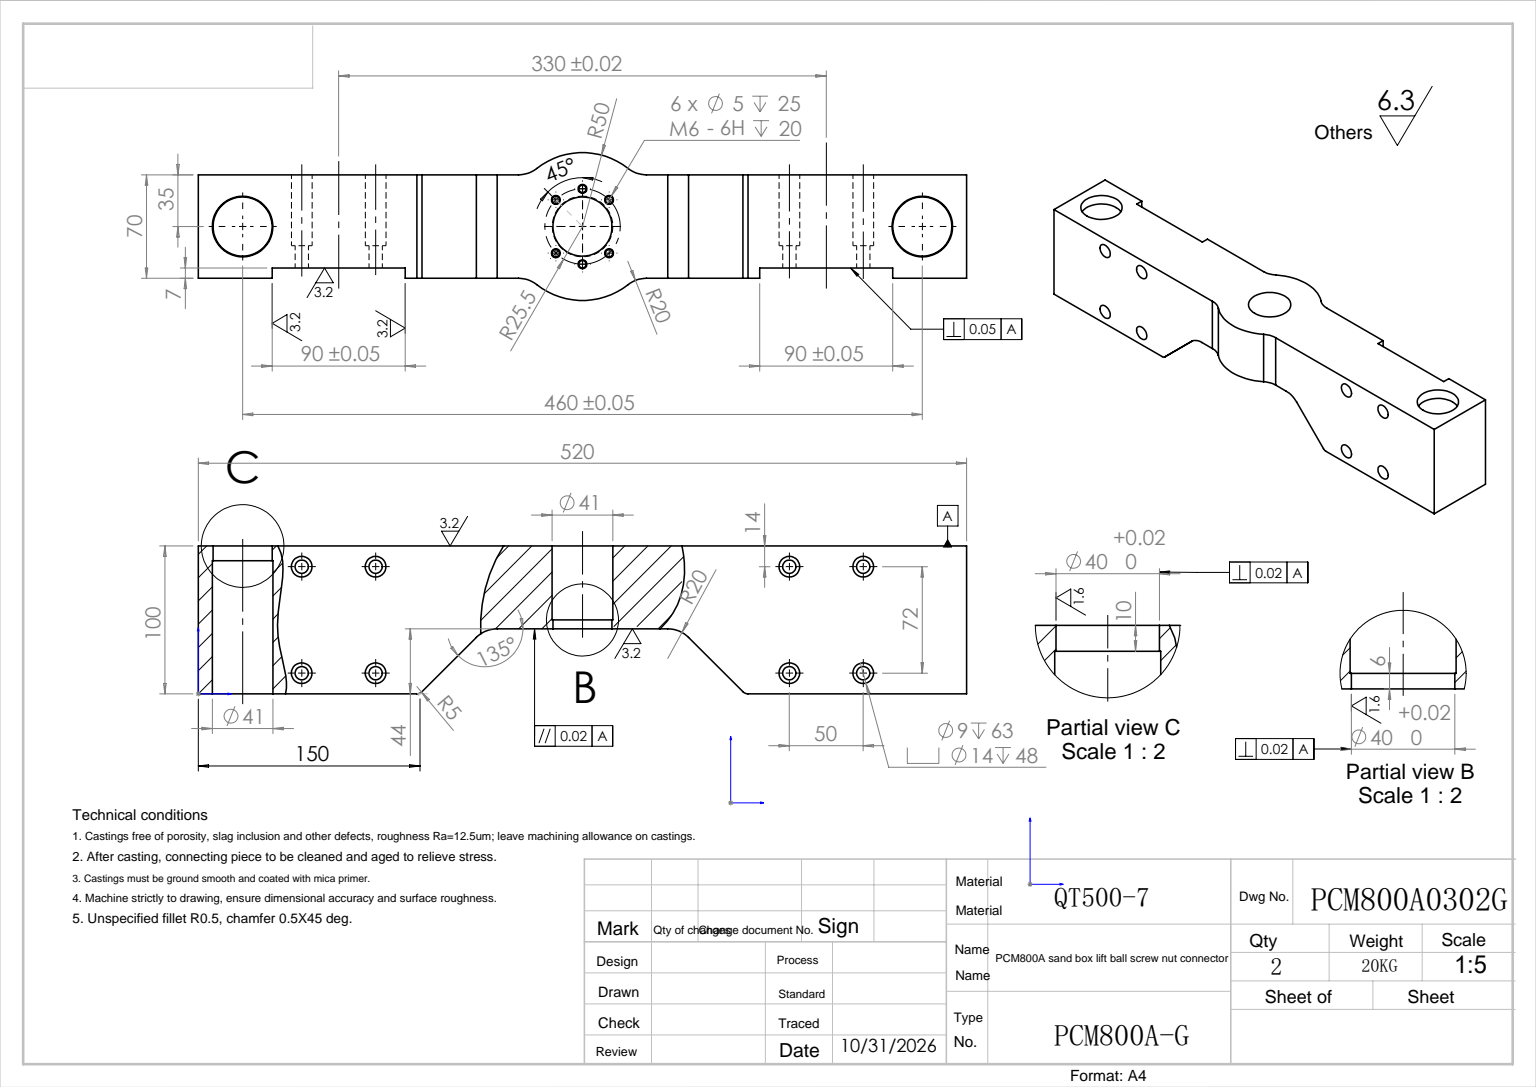
SolidWorks part; units mm, degrees
material "灰铸铁"
ref_plane "前视基准面" through (0, 0, 0) normal (0, 0, 1) x (1, 0, 0)
ref_plane "上视基准面" through (0, 0, 0) normal (0, 1, 0) x (1, 0, 0)
ref_plane "右视基准面" through (0, 0, 0) normal (1, 0, 0) x (0, 0, -1)
sketch "草图1" plane through (0, 0, 0) normal (0, 1, 0) x (1, 0, 0)
  line L0 (0, 70) -> (0, 0)
  line L1 (520, 70) -> (520, 0)
  line L5 (0, 70) -> (50, 70)
  line L6 (50, 70) -> (50, 63)
  line L7 (50, 63) -> (140, 63)
  line L8 (0, 0) -> (216.6987, 0)
  line L9 (260, 0) -> (260, 88.2574) construction
  line L10 (140, 63) -> (140, 70)
  line L11 (140, 70) -> (216.6987, 70)
  line L12 (380, 63) -> (380, 70)
  line L13 (470, 63) -> (380, 63)
  line L14 (470, 70) -> (470, 63)
  line L15 (520, 70) -> (470, 70)
  line L21 (260, 35) -> (280.0863, 35) construction
  line L22 (303.3013, 70) -> (380, 70)
  line L23 (303.3013, 0) -> (520, 0)
  arc A0 (229.0705, -4.2857) -> (290.9295, -4.2857) centre (260, 35) ccw
  arc A1 (290.9295, 74.2857) -> (229.0705, 74.2857) centre (260, 35) ccw
  arc A2 (216.6987, 70) -> (229.0705, 74.2857) centre (216.6987, 90) ccw
  arc A3 (303.3013, 70) -> (290.9295, 74.2857) centre (303.3013, 90) cw
  arc A4 (303.3013, 0) -> (290.9295, -4.2857) centre (303.3013, -20) ccw
  arc A5 (216.6987, 0) -> (229.0705, -4.2857) centre (216.6987, -20) cw
  point P15 (260, 70)
  point P34 (295.7071, 70)
  dimension "D10" = 20
  dimension "D5" = 50
  dimension "D6" = 7
  dimension "D7" = 90
  dimension "D8" = 260
  dimension "D9" = 35
extrude "拉伸1" add sketch "草图1" along normal blind 100
sketch "草图2" plane through (0, 0, 0) normal (0, 0, 1) x (1, 0, 0)
  line L0 (260, 100) -> (260, 0) construction
  line L1 (290.9295, 100) -> (229.0705, 100) construction
  line L2 (229.0705, 0) -> (290.9295, 0) construction
  line L3 (317.7158, 43.9997) -> (202.2842, 43.9997)
  line L5 (0, 0) -> (216.6987, 0) construction
  line L6 (331.8579, 38.1419) -> (370, 0)
  line L8 (188.1421, 38.1419) -> (150, 0)
  line L9 (150, 0) -> (370, 0)
  arc A0 (188.1421, 38.1419) -> (202.2842, 43.9997) centre (202.2842, 23.9997) cw
  arc A1 (331.8579, 38.1419) -> (317.7158, 43.9997) centre (317.7158, 23.9997) ccw
  point P6 (326, 43.9997)
  point P9 (194, 43.9997)
  point P13 (194, 43.9997)
  point P18 (326, 43.9997)
  point P20 (260, 43.9997)
  dimension "D3" = 56.0003
  dimension "D4" = 20
  dimension "D1" = 66
  dimension "D2" = 110
extrude "切除-拉伸1" cut sketch "草图2" against normal through all and the other way through all
sketch "草图3" plane through (0, 43.9997, 0) normal (0, -1, 0) x (1, 0, 0)
  circle A0 centre (260, -35) radius 20
extrude "切除-拉伸2" cut sketch "草图3" against normal through all
ref_plane "基准面1" through (260, 0, 0) normal (1, 0, 0) x (0, 0, -1)
sketch "草图7" plane through (0, 0, -63) normal (0, 0, -1) x (-1, 0, 0)
  line L0 (-425, 100) -> (-425, 0) construction
  line L1 (-470, 100) -> (-380, 100) construction
  line L2 (-470, 0) -> (-380, 0) construction
  line L3 (-470, 50) -> (-380, 50) construction
  line L4 (-470, 100) -> (-470, 0) construction
  line L5 (-380, 100) -> (-380, 0) construction
  line L6 (-450, 86) -> (-400, 86) construction
  line L7 (-400, 86) -> (-400, 14) construction
  line L8 (-400, 14) -> (-450, 14) construction
  line L9 (-450, 14) -> (-450, 86) construction
  circle A0 centre (-450, 86) radius 4.5
  circle A1 centre (-400, 86) radius 4.5
  circle A2 centre (-400, 14) radius 4.5
  circle A3 centre (-450, 14) radius 4.5
  dimension "D1" = 36
  dimension "D2" = 36
  dimension "D3" = 25
  dimension "D4" = 25
extrude "切除-拉伸4" cut sketch "草图7" against normal through all
sketch "草图8" plane through (0, 0, 0) normal (0, 0, 1) x (1, 0, 0)
  circle A0 centre (400, 86) radius 7
  circle A1 centre (450, 86) radius 7
  circle A2 centre (450, 14) radius 7
  circle A3 centre (400, 14) radius 7
extrude "切除-拉伸5" cut sketch "草图8" against normal blind 48
mirror "镜向2" about plane through (260, 0, 0) normal (1, 0, 0) of "切除-拉伸4", "切除-拉伸5"
sketch "草图12" plane through (0, 43.9997, 0) normal (0, -1, 0) x (1, 0, 0)
  line L0 (241.9688, -16.9688) -> (260, -35) construction
  line L1 (260, -35) -> (260, -9.5) construction
  line L2 (260, -35) -> (278.0312, -16.9688) construction
  line L3 (260, -35) -> (278.0312, -53.0312) construction
  line L4 (260, -35) -> (260, -60.5) construction
  line L5 (260, -35) -> (241.9688, -53.0312) construction
  circle A0 centre (260, -35) radius 25.5 construction
  circle A1 centre (260, -9.5) radius 1
  circle A2 centre (241.9688, -16.9688) radius 1
  circle A3 centre (278.0312, -16.9688) radius 1
  circle A4 centre (241.9688, -53.0312) radius 1
  circle A5 centre (260, -60.5) radius 1
  circle A6 centre (278.0312, -53.0312) radius 1
  dimension "D1" = 45
  dimension "D5" = 2
  dimension "D6" = 2
  dimension "D7" = 2
  dimension "D8" = 2
  dimension "D9" = 2
  dimension "D10" = 2
  dimension "D2" = 45
  dimension "D3" = 45
  dimension "D4" = 45
sketch "草图13" plane through (0, 100, 0) normal (0, 1, 0) x (1, 0, 0)
  line L0 (0, 70) -> (0, 0) construction
  line L1 (0, 0) -> (216.6987, 0) construction
  line L2 (520, 0) -> (520, 70) construction
  line L3 (520, 70) -> (470, 70) construction
  circle A0 centre (30, 35) radius 20
  circle A1 centre (490, 35) radius 20
  point P8 (520, 35)
  point P11 (495, 70)
  dimension "D1" = 30
  dimension "D2" = 35
  dimension "D3" = 30
  dimension "D4" = 35
extrude "切除-拉伸7" cut sketch "草图13" against normal through all
extrude "切除-拉伸8" cut sketch "草图12" against normal blind 10
hole_wizard "M6 螺纹孔1" positions "草图17" profile "草图16" tap size "M6" standard "GB"
sketch "草图17" plane through (0, 43.9997, 0) normal (0, -1, 0) x (1, 0, 0)
  point P0 (260, -9.5)
  point P1 (241.9688, -16.9688)
  point P3 (278.0312, -16.9688)
  point P5 (278.0312, -53.0312)
  point P7 (260, -60.5)
  point P9 (241.9688, -53.0312)
sketch "草图16" plane through (260, 43.9997, -9.5) normal (1, 0, 0) x (0, 0, -1)
  line L0 (0, 0) -> (0, 26.5022)
  line L1 (0, 26.5022) -> (2.5, 25)
  line L2 (2.5, 25) -> (2.5, 20)
  line L3 (2.5, 20) -> (3, 20)
  line L4 (3, 20) -> (3, 0)
  line L5 (3, 0) -> (0, 0)
  line L10 (0, 26.5022) -> (-2.5, 25) construction
  line L11 (0, -6.35) -> (0, 107.95) construction
  dimension "螺纹孔钻头直径" = 5
  dimension "螺纹孔钻头深度" = 25
  dimension "螺纹主直径" = 6
  dimension "螺纹深度" = 20
  dimension "导头角度" = 118
sketch "草图18" plane through (0, 0, 0) normal (0, -1, 0) x (1, 0, 0)
  circle A0 centre (30, -35) radius 20.5
  circle A1 centre (490, -35) radius 20.5
  dimension "D1" = 41
  dimension "D2" = 41
extrude "切除-拉伸9" cut sketch "草图18" against normal blind 90
sketch "草图19" plane through (0, 100, 0) normal (0, 1, 0) x (1, 0, 0)
  circle A0 centre (260, 35) radius 20.5
  dimension "D1" = 41
extrude "切除-拉伸10" cut sketch "草图19" against normal blind 50
fillet "圆角1" radius 5 2 edges at (370, 0, -35) (150, 0, -35)
